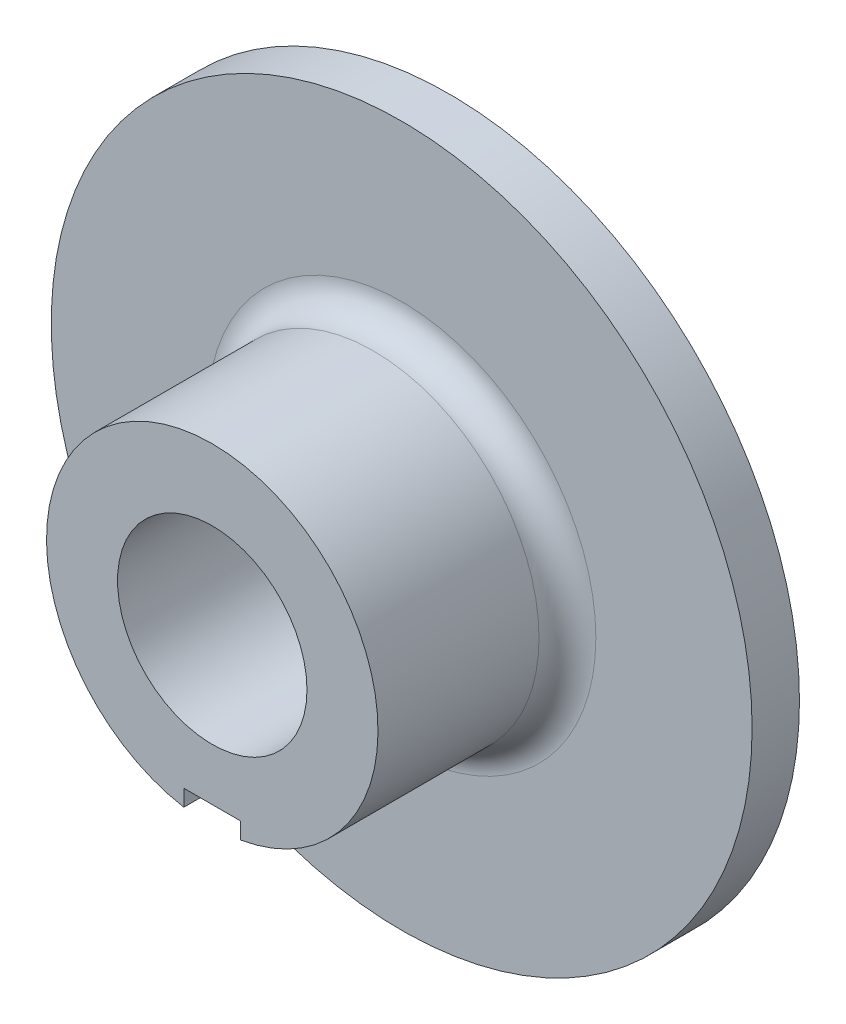
SolidWorks part; units mm, degrees
ref_plane "Front Plane" through (0, 0, 0) normal (0, 0, 1) x (1, 0, 0)
ref_plane "Top Plane" through (0, 0, 0) normal (0, 1, 0) x (1, 0, 0)
ref_plane "Right Plane" through (0, 0, 0) normal (1, 0, 0) x (0, 0, -1)
sketch "Sketch1" plane through (0, 0, 0) normal (0, 0, 1) x (1, 0, 0)
  circle A0 centre (0, 0) radius 37
  dimension "D1" = 74
extrude "Boss-Extrude1" add sketch "Sketch1" along normal blind 5
sketch "Sketch2" plane through (0, 0, 5) normal (0, 0, 1) x (1, 0, 0)
  circle A0 centre (0, 0) radius 17.5
  circle A1 centre (0, 0) radius 10
  dimension "D1" = 35
  dimension "D2" = 20
extrude "Boss-Extrude2" add sketch "Sketch2" along normal blind 20
sketch "Sketch3" plane through (0, 0, 25) normal (0, 0, 1) x (1, 0, 0)
  circle A0 centre (0, 0) radius 10
extrude "Cut-Extrude1" cut sketch "Sketch3" against normal through all
fillet "Fillet1" radius 3 1 edges at (17.5, 0, 5)
sketch "Sketch4" plane through (0, 0, 25) normal (0, 0, 1) x (1, 0, 0)
  line L0 (0, 0) -> (0, -17.5) construction
  line L1 (-3, -19.5) -> (3, -19.5)
  line L2 (-3, -19.5) -> (-3, -15.5)
  line L3 (-3, -15.5) -> (3, -15.5)
  line L4 (3, -19.5) -> (3, -15.5)
  line L5 (-3, -19.5) -> (3, -15.5) construction
  line L6 (-3, -15.5) -> (3, -19.5) construction
  circle A0 centre (0, 0) radius 17.5 construction
  point P0 (0, -17.5)
  dimension "D1" = 4
  dimension "D2" = 6
extrude "Cut-Extrude2" cut sketch "Sketch4" against normal offset from surface (17 mm away) 3 up to face at (20.5, 0, 5)
